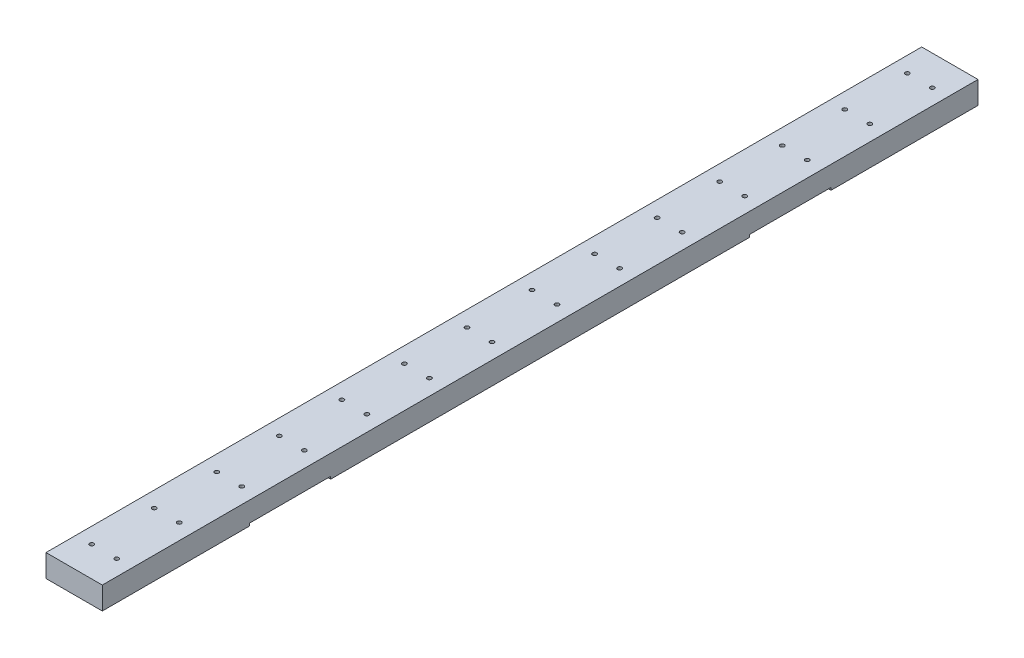
from build123d import *

# Parameters (mm, degrees)
SKETCH1_W             = 45
SKETCH1_H             = 18
BOSS_EXTRUDE1_DEPTH   = 350
M4_TAPPED_HOLE1_D     = 3.3
M4_TAPPED_HOLE1_DEPTH = 10.1
M4_TAPPED_HOLE1_TIP   = 0.991420021
M4_TAPPED_HOLE3_D     = 3.3
SKETCH10_W            = 45
SKETCH10_H            = 65
CUT_EXTRUDE3_DEPTH    = 2
M4_TAPPED_HOLE2_D     = 3.3
M4_TAPPED_HOLE2_DEPTH = 10.1
M4_TAPPED_HOLE2_TIP   = 0.991420021


with BuildPart() as part:
    # Sketch1 → Boss-Extrude1 (new, symmetric)
    with BuildSketch(Plane.XY):
        Rectangle(SKETCH1_W, SKETCH1_H)
    extrude(amount=BOSS_EXTRUDE1_DEPTH, both=True)

    # M4 Tapped Hole1
    with Locations(Plane.ZY.offset(22.5)):
        with Locations((-345, 0), (-300, 0), (-250, 0), (-200, 0), (-150, 0), (-100, 0), (-50, 0), (0, 0), (50, 0), (100, 0), (150, 0), (200, 0), (250, 0), (300, 0), (345, 0)):
            Hole(M4_TAPPED_HOLE1_D / 2, depth=M4_TAPPED_HOLE1_DEPTH)
            with Locations((0, 0, -(M4_TAPPED_HOLE1_DEPTH + M4_TAPPED_HOLE1_TIP / 2))):  # 118° drill point
                Cone(0, M4_TAPPED_HOLE1_D / 2, M4_TAPPED_HOLE1_TIP, mode=Mode.SUBTRACT)

    # M4 Tapped Hole3 (through all)
    with Locations(Plane(origin=(0, -9, 0), x_dir=(-1, 0, 0), z_dir=(0, -1, 0))):
        with Locations((10, -176), (-10, -176), (10, -126), (-10, -126), (10, -226), (-10, -226), (10, -276), (-10, -76), (10, -76), (-10, -276), (10, -326), (-10, -326), (10, 176), (-10, 176), (10, 226), (-10, 226), (10, 326), (-10, 326), (-10, 276), (10, 276), (10, 126), (-10, 126), (-10, 76), (10, 76), (10, 26), (-10, 26), (10, -26), (-10, -26)):
            Hole(M4_TAPPED_HOLE3_D / 2)

    # Sketch10 → Cut-Extrude3 (cut)
    with BuildSketch(Plane.XZ.offset(9)):
        with Locations((0, 200)):
            Rectangle(SKETCH10_W, SKETCH10_H)
        with Locations((0, -200)):
            Rectangle(SKETCH10_W, SKETCH10_H)
    extrude(amount=-CUT_EXTRUDE3_DEPTH, mode=Mode.SUBTRACT)

    # M4 Tapped Hole2
    with Locations(Plane(origin=(0, -7, 0), x_dir=(-1, 0, 0), z_dir=(0, -1, 0))):
        with Locations((9.5, -220), (-10.5, -220), (-10.5, -180), (9.5, -180), (9.5, 180), (-10.5, 180), (-10.5, 220), (9.5, 220)):
            Hole(M4_TAPPED_HOLE2_D / 2, depth=M4_TAPPED_HOLE2_DEPTH)
            with Locations((0, 0, -(M4_TAPPED_HOLE2_DEPTH + M4_TAPPED_HOLE2_TIP / 2))):  # 118° drill point
                Cone(0, M4_TAPPED_HOLE2_D / 2, M4_TAPPED_HOLE2_TIP, mode=Mode.SUBTRACT)


solid = part.part
